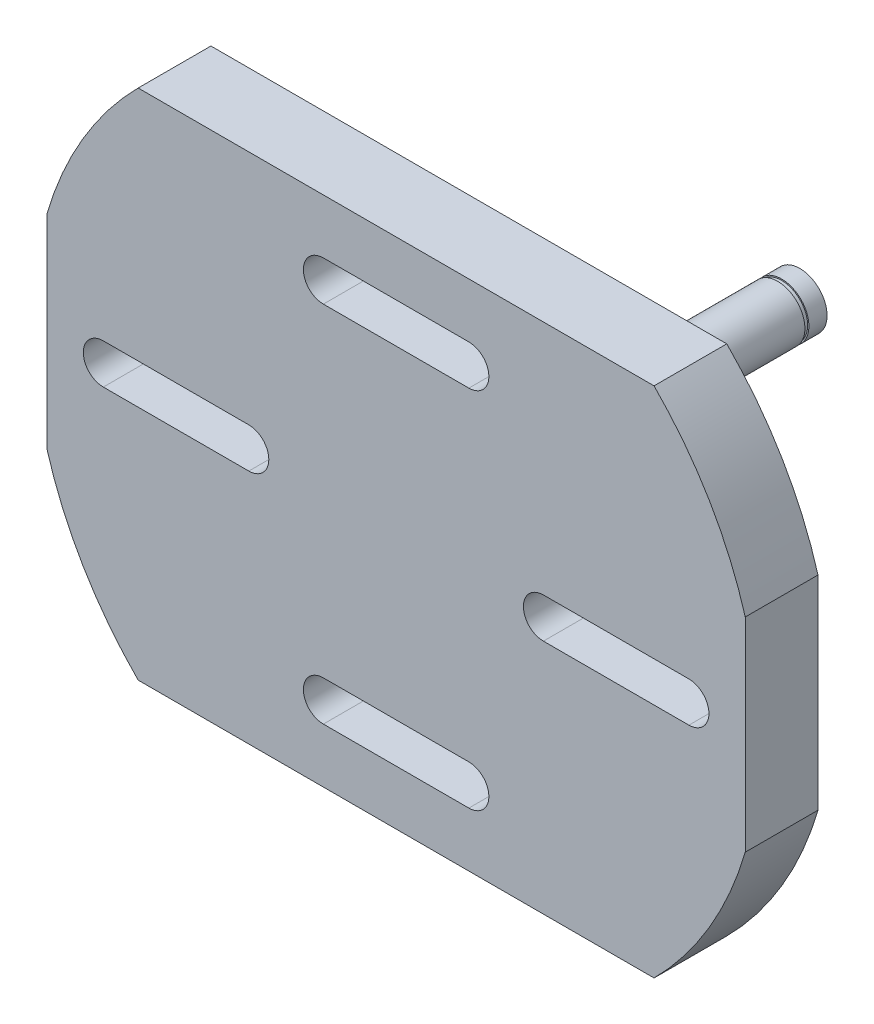
from build123d import *

# Parameters (mm, degrees)
CUT_EXTRUDE_1_DEPTH  = 169.169557293
SKETCH_4_OUTSIDE_W   = 262.768
SKETCH_4_OUTSIDE_H   = 262.768
SKETCH_4_OUTSIDE_W_2 = 192
SKETCH_4_OUTSIDE_H_2 = 141
CUT_EXTRUDE_2_DEPTH  = 169.169557293


with BuildPart() as part:
    # 草图1 → 旋转1 (revolve)
    with BuildSketch(Plane(origin=(0, 0, 0), x_dir=(1, 0, 0), z_dir=(0, 1, 0))):
        Polygon((0, 111), (-7.5, 111), (-7.5, 106), (-7.15, 106), (-7.15, 104.9), (-7.5, 104.9), (-7.5, 60), (-10, 60), (-10, 55), (-30, 55), (-30, 20), (-100, 20), (-100, 0), (0, 0), align=None)
    revolve(axis=Axis((0, 0, 0), (0, 0, 1)))

    # 草图3 → 切除-拉伸1 (cut, through all)
    with BuildSketch(Plane(origin=(0, 0, -20), x_dir=(-1, 0, 0), z_dir=(0, 0, -1))):
        with BuildLine():
            Line((-20, 55.5), (20, 55.5))
            ThreePointArc((20, 55.5), (25.5, 50), (20, 44.5))
            Line((20, 44.5), (-20, 44.5))
            ThreePointArc((-20, 44.5), (-25.5, 50), (-20, 55.5))
        make_face()
        with BuildLine():
            Line((-40.5, -5.5), (-80.5, -5.5))
            ThreePointArc((-80.5, -5.5), (-86, 0), (-80.5, 5.5))
            Line((-80.5, 5.5), (-40.5, 5.5))
            ThreePointArc((-40.5, 5.5), (-35, 0), (-40.5, -5.5))
        make_face()
    cut_extrude_1 = extrude(amount=-CUT_EXTRUDE_1_DEPTH, mode=Mode.SUBTRACT)

    # 镜向1: 切除-拉伸1 across plane
    add(cut_extrude_1.mirror(Plane(origin=(0, 0, 0), x_dir=(0, 0, 1), z_dir=(1, 0, 0))), mode=Mode.SUBTRACT)

    # 镜向2: 切除-拉伸1 across plane
    add(cut_extrude_1.mirror(Plane.ZX), mode=Mode.SUBTRACT)

    # 草图4 outside → 切除-拉伸2 (cut, through all)
    with BuildSketch(Plane(origin=(0, 0, -20), x_dir=(-1, 0, 0), z_dir=(0, 0, -1))):
        Rectangle(SKETCH_4_OUTSIDE_W, SKETCH_4_OUTSIDE_H)
        Rectangle(SKETCH_4_OUTSIDE_W_2, SKETCH_4_OUTSIDE_H_2, mode=Mode.SUBTRACT)
    extrude(amount=-CUT_EXTRUDE_2_DEPTH, mode=Mode.SUBTRACT)


solid = part.part
